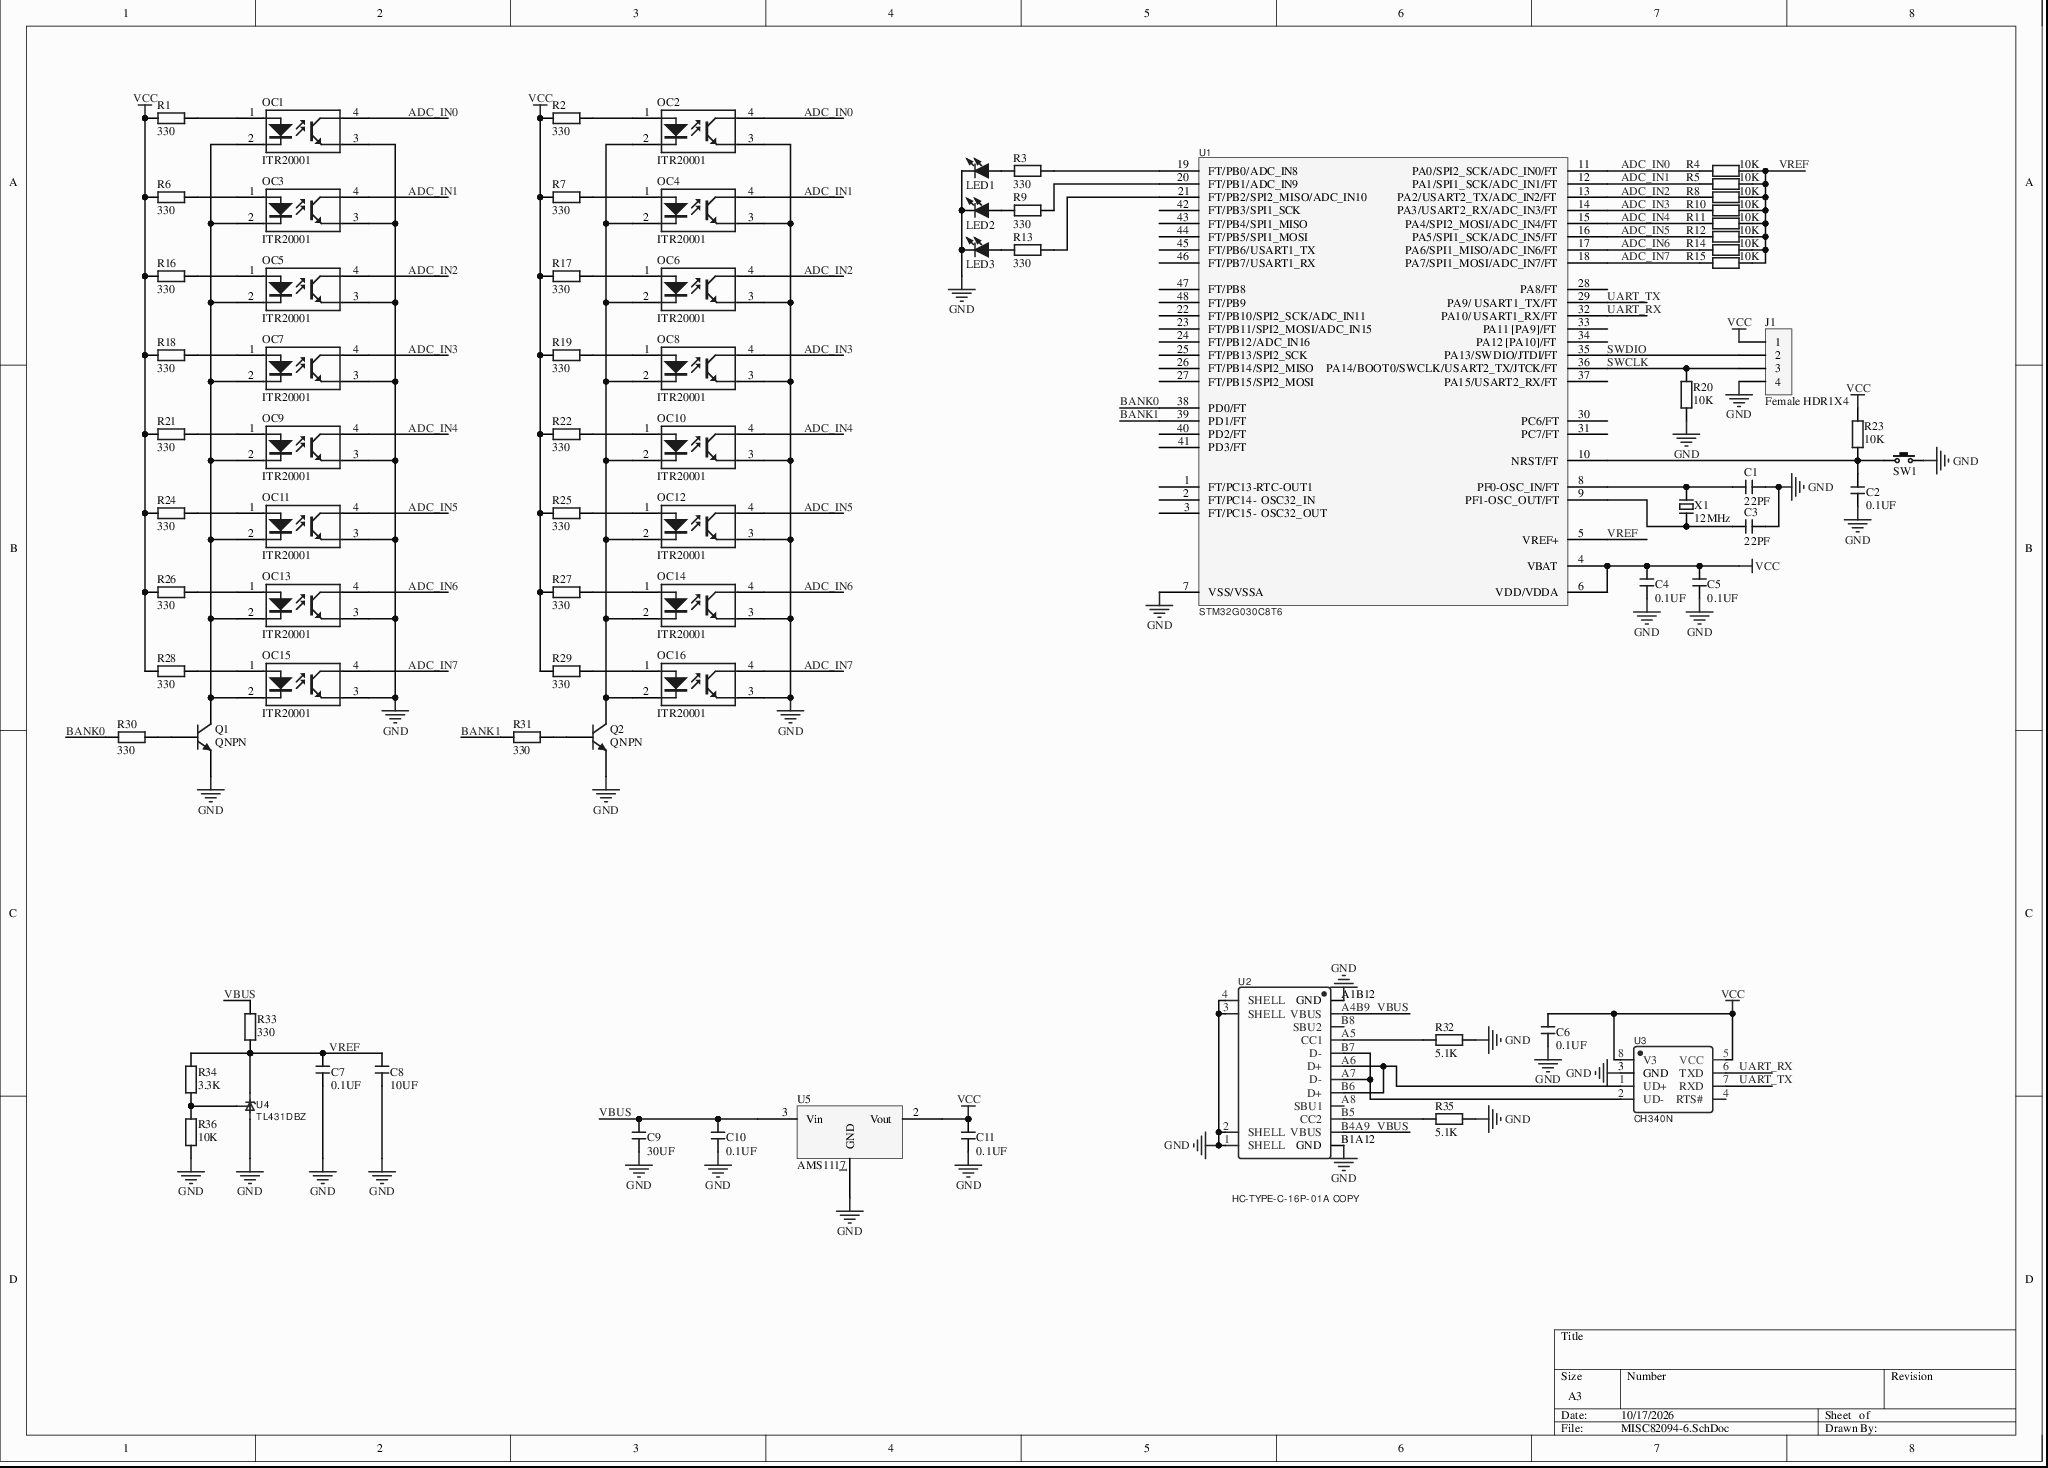
[diagram p0: MISC82094-6.SchDoc]
# Altium project MISC82094-2.PrjPcb
1 sheet, 76 parts. Net scope: global (net labels, ports and power ports of the same name join across sheets).
Board file: MISC82094.PcbDoc

## Sheet MISC82094-6.SchDoc
size A3

### Parts
C1  22PF  [C 0805_L]
C2  0.1UF  [C 0805_L]
C3  22PF  [C 0805_L]
C4  0.1UF  [C 0805_L]
C5  0.1UF  [C 0805_L]
C6  0.1UF  [C 0805_L]
C7  0.1UF  [C 0805_L]
C8  10UF  [C 1206_L]
C9  30UF  [C 1206_L]
C10  0.1UF  [C 0805_L]
C11  0.1UF  [C 0805_L]
J1  Female HDR1X4  [Fe-HDR1X4/2.54-S]
LED1  Red  [LED 0805G]  (value not drawn)
LED2  Red  [LED 0805G]  (value not drawn)
LED3  Red  [LED 0805G]  (value not drawn)
OC1  ITR20001  [SMD_PC817]
OC2  ITR20001  [SMD_PC817]
OC3  ITR20001  [SMD_PC817]
OC4  ITR20001  [SMD_PC817]
OC5  ITR20001  [SMD_PC817]
OC6  ITR20001  [SMD_PC817]
OC7  ITR20001  [SMD_PC817]
OC8  ITR20001  [SMD_PC817]
OC9  ITR20001  [SMD_PC817]
OC10  ITR20001  [SMD_PC817]
OC11  ITR20001  [SMD_PC817]
OC12  ITR20001  [SMD_PC817]
OC13  ITR20001  [SMD_PC817]
OC14  ITR20001  [SMD_PC817]
OC15  ITR20001  [SMD_PC817]
OC16  ITR20001  [SMD_PC817]
Q1  QNPN  [SOT-23B_N]
Q2  QNPN  [SOT-23B_N]
R1  330  [R 0603_L]
R2  330  [R 0603_L]
R3  330  [R 0603_L]
R4  10K  [R 0805_L]
R5  10K  [R 0805_L]
R6  330  [R 0603_L]
R7  330  [R 0603_L]
R8  10K  [R 0805_L]
R9  330  [R 0603_L]
R10  10K  [R 0805_L]
R11  10K  [R 0805_L]
R12  10K  [R 0805_L]
R13  330  [R 0603_L]
R14  10K  [R 0805_L]
R15  10K  [R 0805_L]
R16  330  [R 0603_L]
R17  330  [R 0603_L]
R18  330  [R 0603_L]
R19  330  [R 0603_L]
R20  10K  [R 0805_L]
R21  330  [R 0603_L]
R22  330  [R 0603_L]
R23  10K  [R 0805_L]
R24  330  [R 0603_L]
R25  330  [R 0603_L]
R26  330  [R 0603_L]
R27  330  [R 0603_L]
R28  330  [R 0603_L]
R29  330  [R 0603_L]
R30  330  [R 0603_L]
R31  330  [R 0603_L]
R32  5.1K  [R 0805_L]
R33  330  [R 0805_L]
R34  3.3K  [R 0805_L]
R35  5.1K  [R 0805_L]
R36  10K  [R 0805_L]
SW1  3x6x5  [TSW SMD-3*6*2.5]  (value not drawn)
U1  STM32G030C8T6  [LQFP48_N]
U2  HC-TYPE-C-16P-01A COPY  [USB-C-SMD_HC-TYPE-C-16P-01A]
U3  CH340N  [SOP8]
U4  TL431DBZ  [SOT-23]
U5  AMS1117  [SOT223]
X1  12MHz  [OSC HC-49S]

### Nets
GND: C1.1 C2.1 C3.2 C4.1 C5.1 C6.1 C7.1 C8.1 C9.1 C10.1 C11.1 J1.4 LED1.2(K) LED2.2(K) LED3.2(K) OC1.3(E) OC2.3(E) OC3.3(E) OC4.3(E) OC5.3(E) OC6.3(E) OC7.3(E) OC8.3(E) OC9.3(E) OC10.3(E) OC11.3(E) OC12.3(E) OC13.3(E) OC14.3(E) OC15.3(E) OC16.3(E) Q1.3(E) Q2.3(E) R20.1 R32.1 R35.1 R36.1 SW1.2 U1.7(VSS/VSSA) U2.1(SHELL) U2.2(SHELL) U2.3(SHELL) U2.4(SHELL) U2.A1B12(GND) U2.B1A12(GND) U3.3(GND) U4.3(A) U5.1(GND)
VCC: C4.2 C5.2 C6.2 C11.2 J1.1 R1.1 R2.1 R6.1 R7.1 R16.1 R17.1 R18.1 R19.1 R21.1 R22.1 R23.2 R24.1 R25.1 R26.1 R27.1 R28.1 R29.1 U1.4(VBAT) U1.6(VDD/VDDA) U3.5(VCC) U3.8(V3) U5.2(Vout)
ADC_IN0: OC1.4(C) OC2.4(C) R4.1 U1.11(PA0/SPI2_SCK/ADC_IN0/FT)
ADC_IN1: OC3.4(C) OC4.4(C) R5.1 U1.12(PA1/SPI1_SCK/ADC_IN1/FT)
ADC_IN2: OC5.4(C) OC6.4(C) R8.1 U1.13(PA2/USART2_TX/ADC_IN2/FT)
ADC_IN3: OC7.4(C) OC8.4(C) R10.1 U1.14(PA3/USART2_RX/ADC_IN3/FT)
ADC_IN4: OC9.4(C) OC10.4(C) R11.1 U1.15(PA4/SPI2_MOSI/ADC_IN4/FT)
ADC_IN5: OC11.4(C) OC12.4(C) R12.1 U1.16(PA5/SPI1_SCK/ADC_IN5/FT)
ADC_IN6: OC13.4(C) OC14.4(C) R14.1 U1.17(PA6/SPI1_MISO/ADC_IN6/FT)
ADC_IN7: OC15.4(C) OC16.4(C) R15.1 U1.18(PA7/SPI1_MOSI/ADC_IN7/FT)
BANK0: R30.1 U1.38(PD0/FT)
BANK1: R31.1 U1.39(PD1/FT)
SWCLK: J1.3 R20.2 U1.36(PA14/BOOT0/SWCLK/USART2_TX/JTCK/FT)
SWDIO: J1.2 U1.35(PA13/SWDIO/JTDI/FT)
UART_RX: U1.32(PA10/_USART1_RX/FT) U3.6(TXD)
UART_TX: U1.29(PA9/_USART1_TX/FT) U3.7(RXD)
VBUS: C9.2 C10.2 R33.2 U2.A4B9(VBUS) U2.B4A9(VBUS) U5.3(Vin)
VREF: C7.2 C8.2 R4.2 R5.2 R8.2 R10.2 R11.2 R12.2 R14.2 R15.2 R33.1 R34.2 U1.5(VREF+) U4.2(K)
NetC1_2: C1.2 U1.8(PF0-OSC_IN/FT) X1.2
NetC2_2: C2.2 R23.1 SW1.1 U1.10(NRST/FT)
NetC3_1: C3.1 U1.9(PF1-OSC_OUT/FT) X1.1
NetLED1_1: LED1.1(A) R3.1
NetLED2_1: LED2.1(A) R9.1
NetLED3_1: LED3.1(A) R13.1
NetOC1_1: OC1.1(A) R1.2
NetOC1_2: OC1.2(K) OC3.2(K) OC5.2(K) OC7.2(K) OC9.2(K) OC11.2(K) OC13.2(K) OC15.2(K) Q1.1(C)
NetOC2_1: OC2.1(A) R2.2
NetOC2_2: OC2.2(K) OC4.2(K) OC6.2(K) OC8.2(K) OC10.2(K) OC12.2(K) OC14.2(K) OC16.2(K) Q2.1(C)
NetOC3_1: OC3.1(A) R6.2
NetOC4_1: OC4.1(A) R7.2
NetOC5_1: OC5.1(A) R16.2
NetOC6_1: OC6.1(A) R17.2
NetOC7_1: OC7.1(A) R18.2
NetOC8_1: OC8.1(A) R19.2
NetOC9_1: OC9.1(A) R21.2
NetOC10_1: OC10.1(A) R22.2
NetOC11_1: OC11.1(A) R24.2
NetOC12_1: OC12.1(A) R25.2
NetOC13_1: OC13.1(A) R26.2
NetOC14_1: OC14.1(A) R27.2
NetOC15_1: OC15.1(A) R28.2
NetOC16_1: OC16.1(A) R29.2
NetQ1_2: Q1.2(B) R30.2
NetQ2_2: Q2.2(B) R31.2
NetR3_2: R3.2 U1.19(FT/PB0/ADC_IN8)
NetR9_2: R9.2 U1.20(FT/PB1/ADC_IN9)
NetR13_2: R13.2 U1.21(FT/PB2/SPI2_MISO/ADC_IN10)
NetR32_2: R32.2 U2.A5(CC1)
NetR34_1: R34.1 R36.2 U4.1(REF)
NetR35_2: R35.2 U2.B5(CC2)
NetU2_A6: U2.A6(D+) U2.B6(D+) U3.1(UD+)
NetU2_A7: U2.A7(D-) U2.B7(D-) U3.2(UD-)

Not connected (* = marked no-connect by the designer): U1 1(FT/PC13-RTC-OUT1) 2(FT/PC14-__OSC32_IN) 3(FT/PC15-__OSC32_OUT) 22(FT/PB10/SPI2_SCK/ADC_IN11) 23(FT/PB11/SPI2_MOSI/ADC_IN15) 24(FT/PB12/ADC_IN16) 25(FT/PB13/SPI2_SCK) 26(FT/PB14/SPI2_MISO) 27(FT/PB15/SPI2_MOSI) 28(PA8/FT) 30(PC6/FT) 31(PC7/FT) 33(PA11_[PA9]/FT) 34(PA12_[PA10]/FT) 37(PA15/USART2_RX/FT) 40(PD2/FT) 41(PD3/FT) 42(FT/PB3/SPI1_SCK) 43(FT/PB4/SPI1_MISO) 44(FT/PB5/SPI1_MOSI) 45(FT/PB6/USART1_TX) 46(FT/PB7/USART1_RX) 47(FT/PB8) 48(FT/PB9); U2 A8(SBU1)* B8(SBU2)*; U3 4(RTS#)*

### Library data of the parts
C1-C11 = C: SMD capacitor; BOM名称: Non-polar SMD capacitor
LED1-LED3 = LED-SMD: SMD LED; BOM名称: SMD LED
OC1-OC16 = PC817: Linear optocoupler
Q1 Q2 = QNPN: NPN Bipolar Transistor; Published: 8-Jun-2000; LatestRevisionDate: 29-May-2009; LatestRevisionNote: IPC-7351 Footprint Added.; PackageVersion: Aug-1999; PackageReference: SOT-23B; PackageDescription: 3-Pin SOT-23 Package 0.95 mm Pitch, 2.4 mm Lead Span; Publisher: Altium Limited
R1-R36 = R: SMD resistor; BOM名称: SMD resistor
SW1 = TSW 3x6: 3x6 tact switch; BOM名称: 3x6 tact switch
U5 = AMS1117: Three-terminal voltage regulator
X1 = XTAL-2P: 2-pin passive crystal oscillator; BOM名称: 2-pin passive crystal oscillator